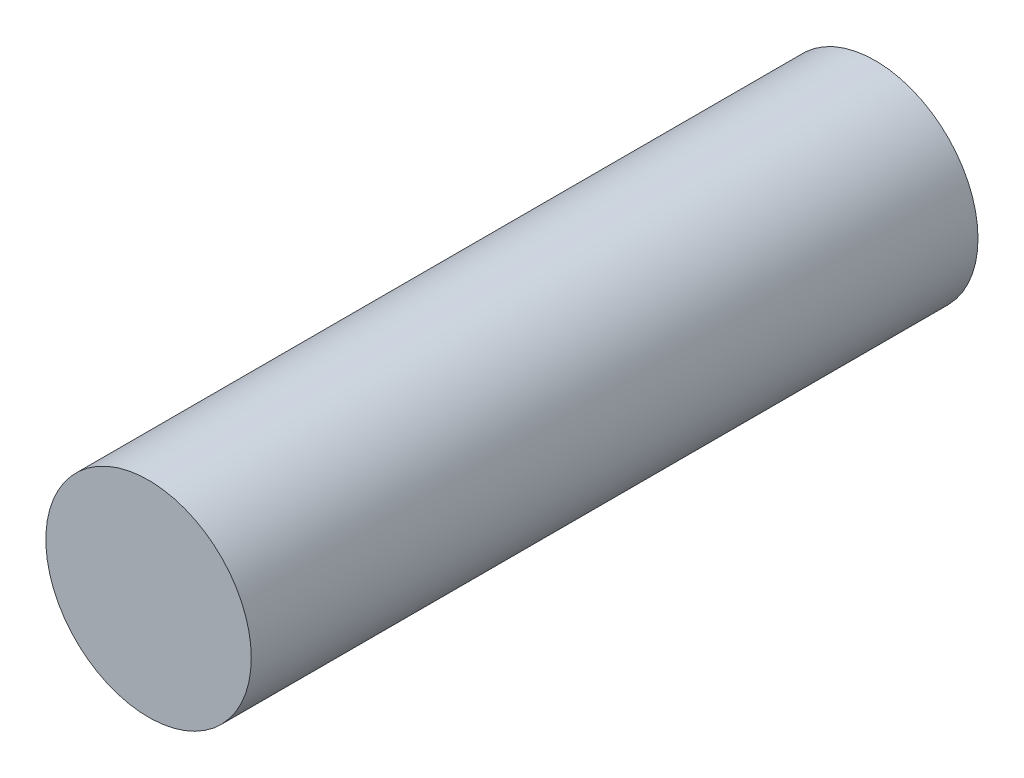
from build123d import *

# Parameters (mm, degrees)
SKETCH1_R           = 3.674588618
BOSS_EXTRUDE1_DEPTH = 13


with BuildPart() as part:
    # Sketch1 → Boss-Extrude1 (new, symmetric)
    with BuildSketch(Plane.XY):
        with Locations((-27.065651732, 16.288746435)):
            Circle(SKETCH1_R)
    extrude(amount=BOSS_EXTRUDE1_DEPTH, both=True)


solid = part.part
